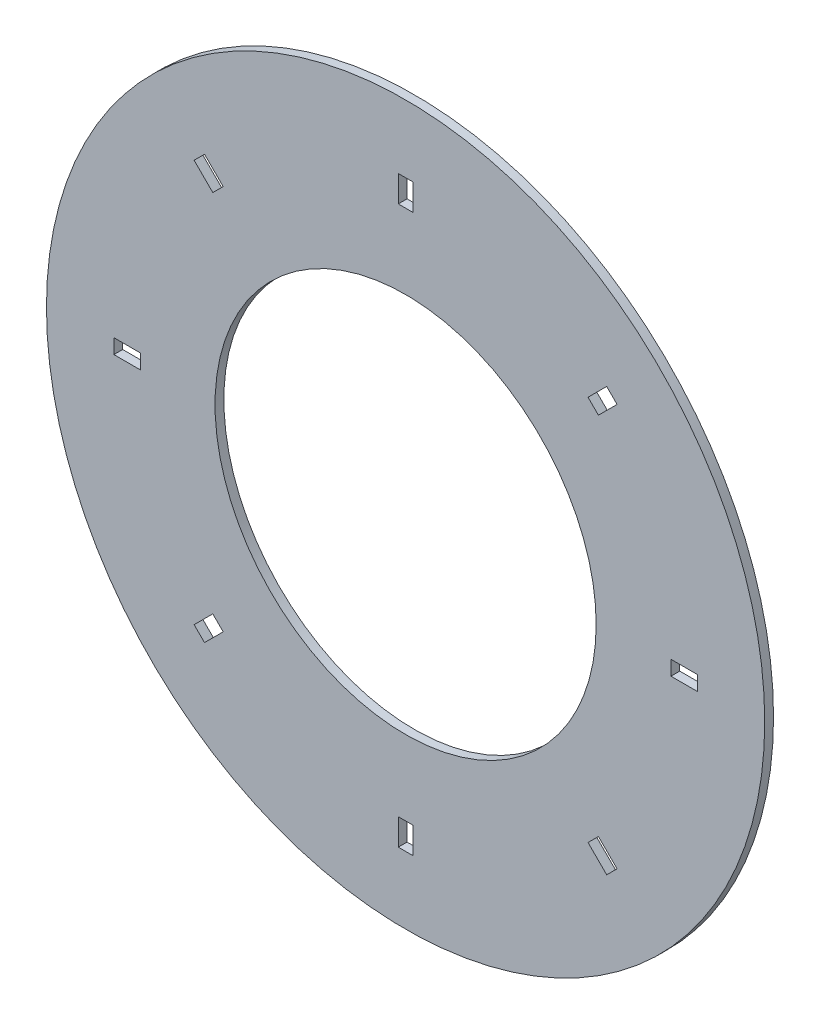
SolidWorks part; units mm, degrees
ref_plane "前视基准面" through (0, 0, 0) normal (0, 0, 1) x (1, 0, 0)
ref_plane "上视基准面" through (0, 0, 0) normal (0, 1, 0) x (1, 0, 0)
ref_plane "右视基准面" through (0, 0, 0) normal (1, 0, 0) x (0, 0, -1)
sketch "草图1" plane through (0, 0, 0) normal (0, 0, 1) x (1, 0, 0)
  circle A0 centre (0, 0) radius 122.5
  circle A1 centre (0, 0) radius 65
  dimension "D1" = 130
  dimension "D2" = 245
extrude "凸台-拉伸1" add sketch "草图1" along normal blind 3
sketch "草图2" plane through (0, 0, 3) normal (0, 0, 1) x (1, 0, 0)
  line L0 (0, 95) -> (0, 0) construction
  line L1 (2.5, 90.5) -> (-2.5, 90.5)
  line L2 (2.5, 90.5) -> (2.5, 99.5)
  line L3 (2.5, 99.5) -> (-2.5, 99.5)
  line L4 (-2.5, 90.5) -> (-2.5, 99.5)
  line L5 (2.5, 90.5) -> (-2.5, 99.5) construction
  line L6 (2.5, 99.5) -> (-2.5, 90.5) construction
  point P0 (0, 95)
  dimension "D1" = 5
  dimension "D2" = 9
  dimension "D3" = 95
extrude "切除-拉伸1" cut sketch "草图2" against normal blind 5
pattern_circular "阵列(圆周)1" count 8 over 360 about axis through (0, 0, 0) along (0, 0, 1) of "切除-拉伸1"
